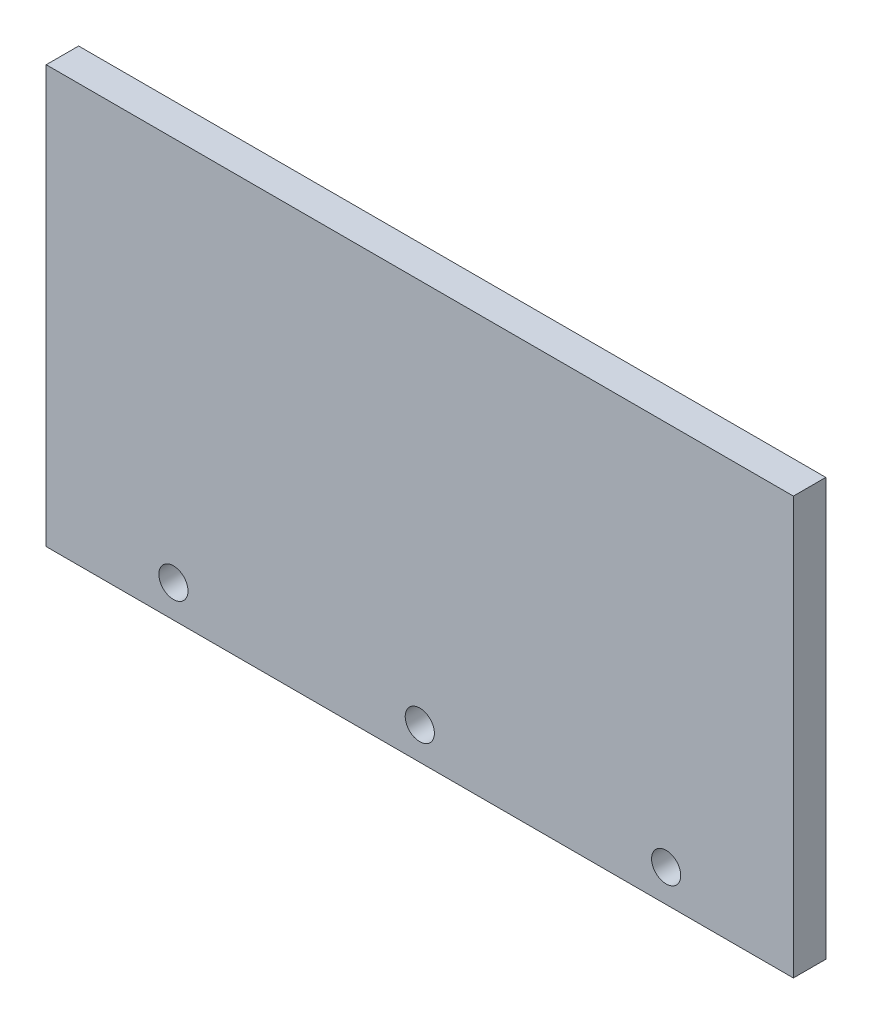
SolidWorks part; units mm, degrees
material "Q235"
ref_plane "Front Plane" through (0, 0, 0) normal (0, 0, 1) x (1, 0, 0)
ref_plane "Top Plane" through (0, 0, 0) normal (0, 1, 0) x (1, 0, 0)
ref_plane "Right Plane" through (0, 0, 0) normal (1, 0, 0) x (0, 0, -1)
sketch "Sketch1" plane through (0, 0, 0) normal (0, 0, 1) x (1, 0, 0)
  line L1 (0, 0) -> (922, 0)
  line L2 (0, 0) -> (0, 515)
  line L3 (0, 515) -> (922, 515)
  line L4 (922, 0) -> (922, 515)
  circle A0 centre (461, 40) radius 18
  circle A1 centre (765, 40) radius 18
  circle A2 centre (157, 40) radius 18
  point P12 (461, 0)
  dimension "D3" = 36
  dimension "D4" = 304
  dimension "D5" = 304
  dimension "D6" = 40
  dimension "D1" = 922
  dimension "D2" = 515
extrude "Boss-Extrude1" add sketch "Sketch1" along normal blind 40
